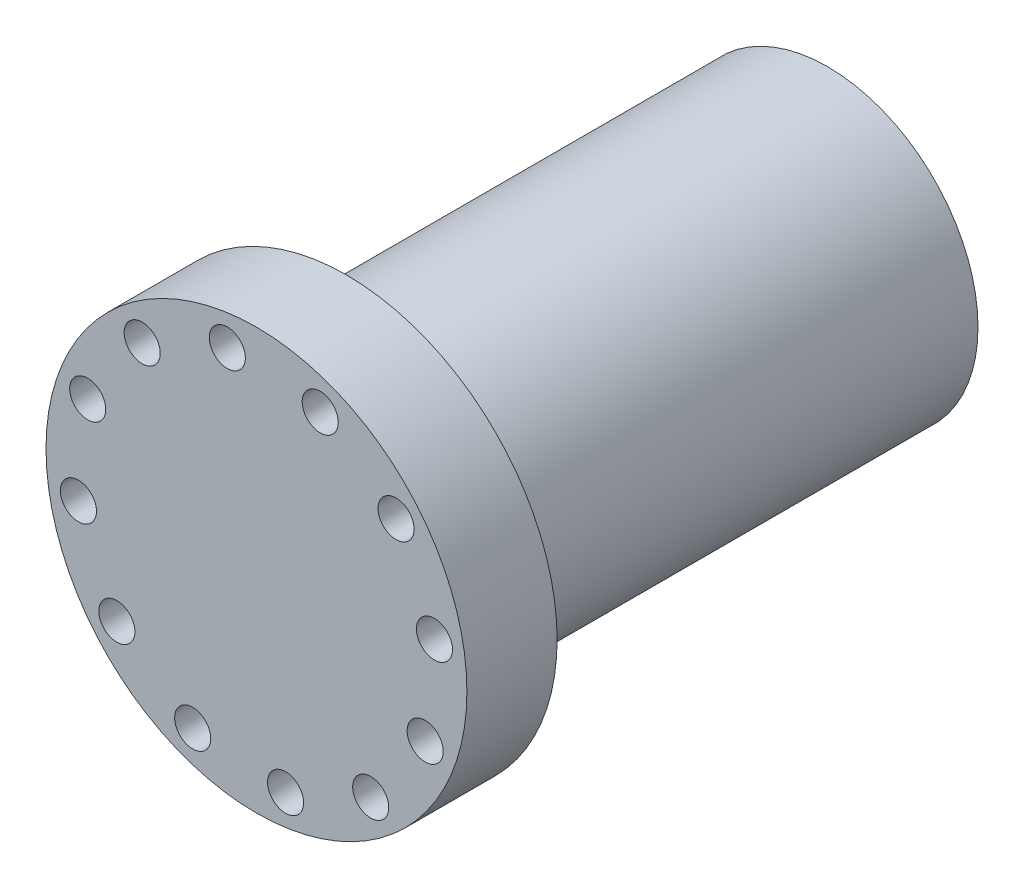
SolidWorks part; units mm, degrees
ref_plane "Front Plane" through (0, 0, 0) normal (0, 0, 1) x (1, 0, 0)
ref_plane "Top Plane" through (0, 0, 0) normal (0, 1, 0) x (1, 0, 0)
ref_plane "Right Plane" through (0, 0, 0) normal (1, 0, 0) x (0, 0, -1)
sketch "Sketch1" plane through (0, 0, 0) normal (0, 0, 1) x (1, 0, 0)
  circle A0 centre (-70, 25) radius 17.5
extrude "Boss-Extrude1" add sketch "Sketch1" along normal blind 7.5
sketch "Sketch2" plane through (0, 0, 0) normal (0, 0, -1) x (-1, 0, 0)
  circle A0 centre (70, 25) radius 12.5
extrude "Boss-Extrude2" add sketch "Sketch2" along normal blind 40
sketch "Sketch3" plane through (0, 0, 7.5) normal (0, 0, 1) x (1, 0, 0)
  circle A0 centre (-81.6083, 15.5002) radius 1.5
  circle A1 centre (-70, 25) radius 15 construction
  circle A2 centre (-84.803, 22.577) radius 1.5
  circle A3 centre (-84.0313, 30.3032) radius 1.5
  circle A4 centre (-79.4998, 36.6083) radius 1.5
  circle A5 centre (-72.423, 39.803) radius 1.5
  circle A6 centre (-64.6968, 39.0313) radius 1.5
  circle A7 centre (-58.3917, 34.4998) radius 1.5
  circle A8 centre (-55.197, 27.423) radius 1.5
  circle A9 centre (-55.9687, 19.6968) radius 1.5
  circle A10 centre (-60.5002, 13.3917) radius 1.5
  circle A11 centre (-67.577, 10.197) radius 1.5
  circle A12 centre (-75.3032, 10.9687) radius 1.5
  dimension "D1" = 3
  dimension "D2" = 30
  dimension "D3" = 12
extrude "Cut-Extrude1" cut sketch "Sketch3" against normal through all and the other way through all
